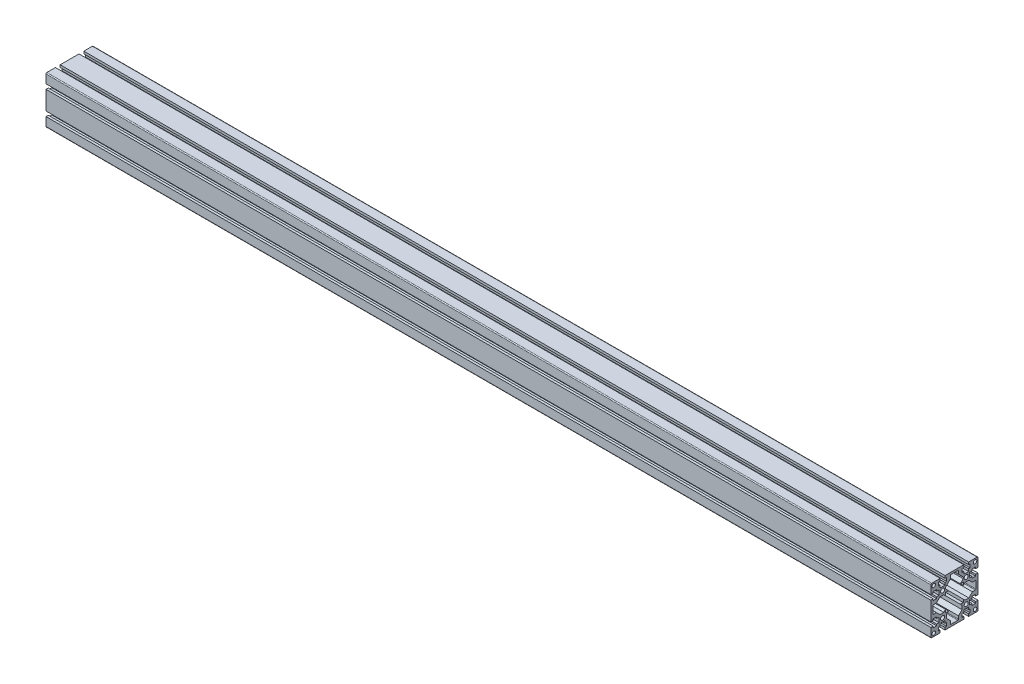
SolidWorks part; units mm, degrees
ref_plane "Front Plane" through (0, 0, 0) normal (0, 0, 1) x (1, 0, 0)
ref_plane "Top Plane" through (0, 0, 0) normal (0, 1, 0) x (1, 0, 0)
ref_plane "Right Plane" through (0, 0, 0) normal (1, 0, 0) x (0, 0, -1)
sketch "草图1" plane through (0, 0, 0) normal (0, 0, 1) x (1, 0, 0)
  line L0 (-530.3448, 0) -> (969.6552, 0)
  dimension "D1" = 1500
other "Aluminum profile 80 X 80G X R1.5(1)"
ref_plane "Plane2" through (-530.3448, 0, 0) normal (1, 0, 0) x (0, 1, 0)
sketch "Sketch1" plane through (-530.3448, 0, 0) normal (1, 0, 0) x (0, 1, 0)
  line L0 (0, 40) -> (0, 0) construction
  line L1 (0, 0) -> (40, 0) construction
  line L2 (-24.05, 40) -> (-24.05, 36)
  line L3 (-38.5, 40) -> (-24.05, 40)
  line L4 (-40, 38.5) -> (-40, 24.05)
  line L5 (-38.5, -40) -> (-24.05, -40)
  line L6 (40, 38.5) -> (40, 24.05)
  line L7 (-24.05, 36) -> (-26.75, 36)
  line L8 (-26.75, 36) -> (-26.75, 30)
  line L9 (-26.75, 30) -> (-24.05, 30)
  line L10 (-24.05, 30) -> (-24.05, 26)
  line L11 (-24.05, 26) -> (-15.95, 26)
  line L12 (-15.95, 26) -> (-15.95, 30)
  line L13 (-15.95, 30) -> (-13.25, 30)
  line L14 (-13.25, 30) -> (-13.25, 36)
  line L15 (-13.25, 36) -> (-15.95, 36)
  line L16 (-15.95, 36) -> (-15.95, 40)
  line L17 (-40, 15.95) -> (-36, 15.95)
  line L18 (-36, 15.95) -> (-36, 13.25)
  line L19 (-15.95, 40) -> (15.95, 40)
  line L20 (-20, 20) -> (-20, 40) construction
  line L21 (20, 20) -> (20, 40) construction
  line L22 (15.95, 36) -> (15.95, 40)
  line L23 (13.25, 36) -> (15.95, 36)
  line L24 (13.25, 30) -> (13.25, 36)
  line L25 (15.95, 30) -> (13.25, 30)
  line L26 (-36, 13.25) -> (-30, 13.25)
  line L27 (-30, 13.25) -> (-30, 15.95)
  line L28 (-26, 15.95) -> (-26, 24.05)
  line L29 (-26, 24.05) -> (-30, 24.05)
  line L30 (-30, 24.05) -> (-30, 26.75)
  line L31 (-30, 26.75) -> (-36, 26.75)
  line L32 (-36, 26.75) -> (-36, 24.05)
  line L33 (-36, 24.05) -> (-40, 24.05)
  line L34 (-30, 15.95) -> (-26, 15.95)
  line L35 (15.95, 26) -> (15.95, 30)
  line L36 (24.05, 26) -> (15.95, 26)
  line L37 (24.05, 30) -> (24.05, 26)
  line L38 (26.75, 30) -> (24.05, 30)
  line L39 (26.75, 36) -> (26.75, 30)
  line L40 (24.05, 36) -> (26.75, 36)
  line L41 (24.05, 40) -> (24.05, 36)
  line L42 (24.05, -40) -> (24.05, -36)
  line L43 (24.05, -36) -> (26.75, -36)
  line L44 (26.75, -36) -> (26.75, -30)
  line L45 (26.75, -30) -> (24.05, -30)
  line L46 (24.05, -30) -> (24.05, -26)
  line L47 (24.05, -26) -> (15.95, -26)
  line L48 (15.95, -26) -> (15.95, -30)
  line L49 (15.95, -30) -> (13.25, -30)
  line L50 (13.25, -30) -> (13.25, -36)
  line L51 (13.25, -36) -> (15.95, -36)
  line L52 (15.95, -36) -> (15.95, -40)
  line L53 (-15.95, -36) -> (-15.95, -40)
  line L54 (-13.25, -36) -> (-15.95, -36)
  line L55 (-13.25, -30) -> (-13.25, -36)
  line L56 (-15.95, -30) -> (-13.25, -30)
  line L57 (-15.95, -26) -> (-15.95, -30)
  line L58 (-24.05, -26) -> (-15.95, -26)
  line L59 (-24.05, -30) -> (-24.05, -26)
  line L60 (-26.75, -30) -> (-24.05, -30)
  line L61 (-26.75, -36) -> (-26.75, -30)
  line L62 (-24.05, -36) -> (-26.75, -36)
  line L63 (-24.05, -40) -> (-24.05, -36)
  line L64 (-30, -15.95) -> (-26, -15.95)
  line L65 (-36, -26.75) -> (-36, -24.05)
  line L66 (-30, -26.75) -> (-36, -26.75)
  line L67 (-30, -24.05) -> (-30, -26.75)
  line L68 (-26, -24.05) -> (-30, -24.05)
  line L69 (-26, -15.95) -> (-26, -24.05)
  line L70 (-30, -13.25) -> (-30, -15.95)
  line L71 (-36, -13.25) -> (-30, -13.25)
  line L72 (-36, -15.95) -> (-36, -13.25)
  line L73 (36, 24.05) -> (40, 24.05)
  line L74 (40, 15.95) -> (36, 15.95)
  line L75 (36, -15.95) -> (36, -13.25)
  line L76 (36, -13.25) -> (30, -13.25)
  line L77 (30, -13.25) -> (30, -15.95)
  line L78 (26, -15.95) -> (26, -24.05)
  line L79 (26, -24.05) -> (30, -24.05)
  line L80 (30, -24.05) -> (30, -26.75)
  line L81 (30, -26.75) -> (36, -26.75)
  line L82 (36, -26.75) -> (36, -24.05)
  line L83 (30, -15.95) -> (26, -15.95)
  line L84 (30, 15.95) -> (26, 15.95)
  line L85 (36, 26.75) -> (36, 24.05)
  line L86 (30, 26.75) -> (36, 26.75)
  line L87 (30, 24.05) -> (30, 26.75)
  line L88 (26, 24.05) -> (30, 24.05)
  line L89 (26, 15.95) -> (26, 24.05)
  line L90 (30, 13.25) -> (30, 15.95)
  line L91 (36, 13.25) -> (30, 13.25)
  line L92 (36, 15.95) -> (36, 13.25)
  line L93 (-36, -15.95) -> (-40, -15.95)
  line L94 (-36, -24.05) -> (-40, -24.05)
  line L95 (36, -15.95) -> (40, -15.95)
  line L96 (36, -24.05) -> (40, -24.05)
  line L97 (-13, 18) -> (-10, 15)
  line L98 (-15, 15) -> (-10, 15)
  line L99 (-15, 15) -> (-15, 10)
  line L100 (-15, -15) -> (-10, -15)
  line L101 (15, 15) -> (15, 10)
  line L102 (-18, 13) -> (-15, 10)
  line L104 (13, 18) -> (10, 15)
  line L105 (13, -18) -> (10, -15)
  line L106 (20, -15) -> (15, -10)
  line L107 (-18, -13) -> (-15, -10)
  line L108 (-13, -18) -> (-10, -15)
  line L109 (15, -10) -> (15, -15)
  line L110 (10, 15) -> (15, 15)
  line L111 (-15, -10) -> (-15, -15)
  line L112 (10, -15) -> (15, -15)
  line L113 (15, 10) -> (20, 15)
  line L235 (24.05, 40) -> (38.5, 40)
  line L249 (-40, 15.95) -> (-40, -15.95)
  line L250 (-20, 20) -> (-26, 20) construction
  line L264 (40, 15.95) -> (40, -15.95)
  line L265 (-13, 24.5) -> (-7, 30.5)
  line L266 (-7, 30.5) -> (-7, 35.5)
  line L267 (7, 35.5) -> (7, 30.5)
  line L268 (7, 30.5) -> (13, 24.5)
  line L269 (-6, -36.5) -> (6, -36.5)
  line L270 (-13, 24.5) -> (-13, 18)
  line L271 (-35.5, 7) -> (-30.5, 7)
  line L272 (-30.5, 7) -> (-24.5, 13)
  line L273 (-24.5, 13) -> (-18, 13)
  line L274 (13, 24.5) -> (13, 18)
  line L275 (-15.95, -40) -> (15.95, -40)
  line L276 (35.5, 7) -> (30.5, 7)
  line L277 (30.5, 7) -> (22.5, 15)
  line L278 (24.05, -40) -> (38.5, -40)
  line L279 (20, 15) -> (22.5, 15)
  line L333 (-13, -24.5) -> (-13, -18)
  line L336 (-13, -24.5) -> (-7, -30.5)
  line L385 (-7, -30.5) -> (-7, -35.5)
  line L386 (-36.5, 6) -> (-36.5, -6)
  line L387 (7, -35.5) -> (7, -30.5)
  line L429 (7, -30.5) -> (13, -24.5)
  line L430 (13, -24.5) -> (13, -18)
  line L494 (20, -15) -> (22.5, -15)
  line L496 (30.5, -7) -> (22.5, -15)
  line L497 (35.5, -7) -> (30.5, -7)
  line L498 (-24.5, -13) -> (-18, -13)
  line L499 (-30.5, -7) -> (-24.5, -13)
  line L500 (-35.5, -7) -> (-30.5, -7)
  line L512 (40, -24.05) -> (40, -38.5)
  line L519 (-40, -24.05) -> (-40, -38.5)
  line L520 (-6, 36.5) -> (6, 36.5)
  line L523 (36.5, 6) -> (36.5, -6)
  circle A0 centre (-20, 20) radius 3.4
  circle A2 centre (20, 20) radius 3.4
  circle A3 centre (20, -20) radius 3.4
  circle A7 centre (-20, -20) radius 3.4
  arc A8 (-38.5, 40) -> (-40, 38.5) centre (-38.5, 38.5) ccw
  arc A9 (-40, -38.5) -> (-38.5, -40) centre (-38.5, -38.5) ccw
  arc A10 (38.5, -40) -> (40, -38.5) centre (38.5, -38.5) ccw
  arc A11 (38.5, 40) -> (40, 38.5) centre (38.5, 38.5) cw
  circle A12 centre (-35, 35) radius 3
  circle A13 centre (35, 35) radius 3
  circle A14 centre (35, -35) radius 3
  arc A15 (-6, 36.5) -> (-7, 35.5) centre (-6, 35.5) ccw
  arc A16 (6, 36.5) -> (7, 35.5) centre (6, 35.5) cw
  arc A17 (-36.5, 6) -> (-35.5, 7) centre (-35.5, 6) cw
  arc A18 (-36.5, -6) -> (-35.5, -7) centre (-35.5, -6) ccw
  arc A19 (36.5, -6) -> (35.5, -7) centre (35.5, -6) cw
  arc A20 (36.5, 6) -> (35.5, 7) centre (35.5, 6) ccw
  arc A21 (6, -36.5) -> (7, -35.5) centre (6, -35.5) ccw
  arc A22 (-6, -36.5) -> (-7, -35.5) centre (-6, -35.5) cw
  point P48 (-20, 20)
  point P97 (0, 0)
  point P104 (-7, 36.5)
  point P185 (40, 40)
  point P187 (40, -40)
  point P188 (-40, -40)
  point P190 (-40, 40)
  dimension "D1" = 80
  dimension "D2" = 80
  dimension "D3" = 20
  dimension "D4" = 8.1
  dimension "D5" = 45
  dimension "D6" = 7
  dimension "D7" = 13.5
  dimension "D8" = 6
  dimension "D12" = 5
  dimension "D13" = 5
  dimension "D14" = 20
  dimension "D18" = 1
  dimension "D19" = 14
  dimension "D15" = 6.8
  dimension "D27" = 45
  dimension "D20" = 1.5
  dimension "D11" = 6
  dimension "D9" = 4
  dimension "D10" = 14
  dimension "D16" = 14
  dimension "D17" = 45
  dimension "D21" = 3.5
  dimension "D22" = 3.5
  dimension "D23" = 73
  dimension "D24" = 30
  dimension "D25" = 30
  dimension "D26" = 45
  dimension "D28" = 5
sketch "Sketch10" plane through (969.6552, 0, 0) normal (1, 0, 0) x (0, 0, -1)
  circle A0 centre (35, -35) radius 3
  circle A1 centre (-35, -35) radius 3 construction
  circle A2 centre (35, 35) radius 3 construction
  dimension "D1" = 6
  dimension "D2" = 70
  dimension "D3" = 70
extrude "Cut-Extrude1" cut sketch "Sketch10" against normal through all
